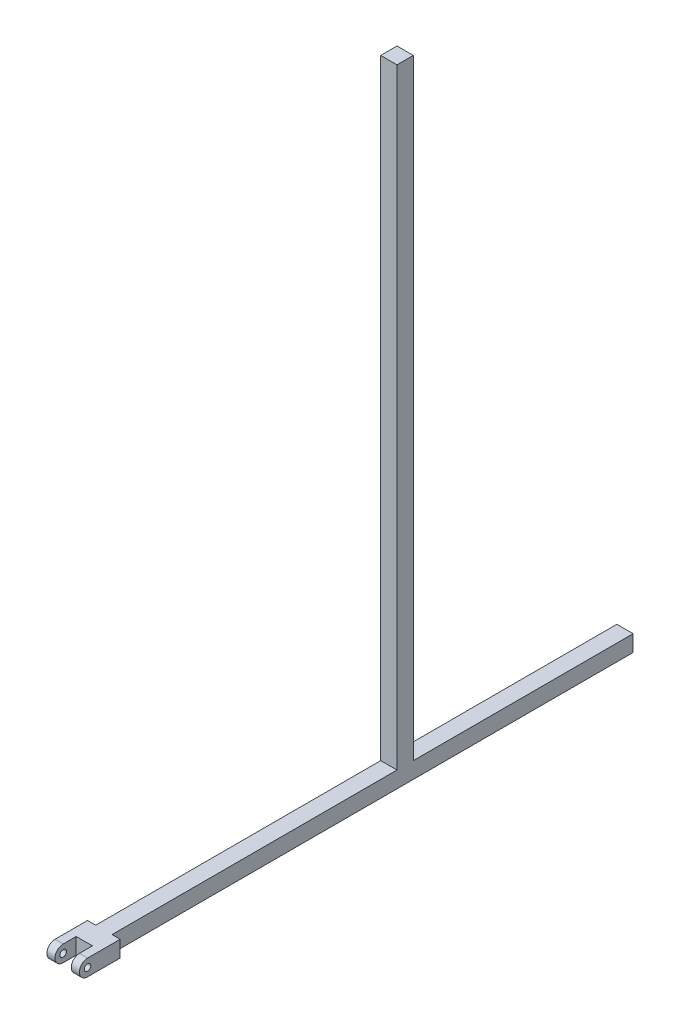
SolidWorks part; units mm, degrees
ref_plane "Front Plane" through (0, 0, 0) normal (0, 0, 1) x (1, 0, 0)
ref_plane "Top Plane" through (0, 0, 0) normal (0, 1, 0) x (1, 0, 0)
ref_plane "Right Plane" through (0, 0, 0) normal (1, 0, 0) x (0, 0, -1)
other "Configuration Table"
sketch "Sketch1" plane through (0, 0, 0) normal (0, 0, 1) x (1, 0, 0)
  line L1 (-2.5, 2.5) -> (2.5, 2.5)
  line L2 (-2.5, 2.5) -> (-2.5, -2.5)
  line L3 (-2.5, -2.5) -> (2.5, -2.5)
  line L4 (2.5, 2.5) -> (2.5, -2.5)
  line L5 (-2.5, 2.5) -> (2.5, -2.5) construction
  line L6 (-2.5, -2.5) -> (2.5, 2.5) construction
  point P0 (0, 0)
  dimension "D1" = 5
  dimension "D2" = 5
extrude "Boss-Extrude1" add sketch "Sketch1" along normal blind 160
sketch "Sketch2" plane through (0, 0, 160) normal (0, 0, 1) x (1, 0, 0)
  line L1 (-5, 2.5) -> (5, 2.5)
  line L2 (-5, 2.5) -> (-5, -2.5)
  line L3 (-5, -2.5) -> (5, -2.5)
  line L4 (5, 2.5) -> (5, -2.5)
  line L5 (-5, 2.5) -> (5, -2.5) construction
  line L6 (-5, -2.5) -> (5, 2.5) construction
  point P0 (0, 0)
  dimension "D1" = 10
  dimension "D2" = 5
extrude "Boss-Extrude2" add sketch "Sketch2" along normal blind 18
sketch "Sketch3" plane through (0, 0, 178) normal (0, 0, 1) x (1, 0, 0)
  line L1 (-2.5, 9.6791) -> (2.5, 9.6791)
  line L2 (-2.5, 9.6791) -> (-2.5, -9.6791)
  line L3 (-2.5, -9.6791) -> (2.5, -9.6791)
  line L4 (2.5, 9.6791) -> (2.5, -9.6791)
  line L5 (-2.5, 9.6791) -> (2.5, -9.6791) construction
  line L6 (-2.5, -9.6791) -> (2.5, 9.6791) construction
  point P0 (0, 0)
  dimension "D1" = 5
extrude "Cut-Extrude1" cut sketch "Sketch3" against normal blind 12
sketch "Sketch4" plane through (5, 0, 0) normal (1, 0, 0) x (0, 0, -1)
  line L0 (-170, 2.5) -> (-170, 12.5754)
  line L1 (-170, 12.5754) -> (-197.274, 12.5754)
  line L2 (-197.274, 12.5754) -> (-202.2181, -13.9989)
  line L3 (-202.2181, -13.9989) -> (-170, -2.5)
  line L4 (-178, -2.5) -> (-178, 2.5) construction
  line L5 (-178, -2.5) -> (-160, -2.5) construction
  circle A0 centre (-170, 0) radius 1
  arc A1 (-170, 2.5) -> (-170, -2.5) centre (-170, 0) ccw
  dimension "D1" = 2
  dimension "D2" = 5
  dimension "D3" = 8
  dimension "D4" = 2.5
extrude "Cut-Extrude2" cut sketch "Sketch4" against normal through all both and the other way through all
sketch "Sketch5" plane through (0, 0, 0) normal (0, 1, 0) x (1, 0, 0)
  line L1 (2.5, -160) -> (2.5, 0) construction
  line L2 (-2.5, -67.5) -> (2.5, -67.5)
  line L3 (-2.5, -67.5) -> (-2.5, -72.5)
  line L4 (-2.5, -72.5) -> (2.5, -72.5)
  line L5 (2.5, -67.5) -> (2.5, -72.5)
  line L6 (-2.5, -67.5) -> (2.5, -72.5) construction
  line L7 (-2.5, -72.5) -> (2.5, -67.5) construction
  point P0 (0, -70)
  dimension "D1" = 5
  dimension "D2" = 70
  dimension "D3" = 5
extrude "Boss-Extrude3" add sketch "Sketch5" along normal blind 190
sketch "Sketch6" plane through (-2.5, 0, 0) normal (1, 0, 0) x (0, 0, -1)
  line L0 (-170, 0) -> (-169, 0) construction
  circle A0 centre (-170, 0) radius 1 construction
